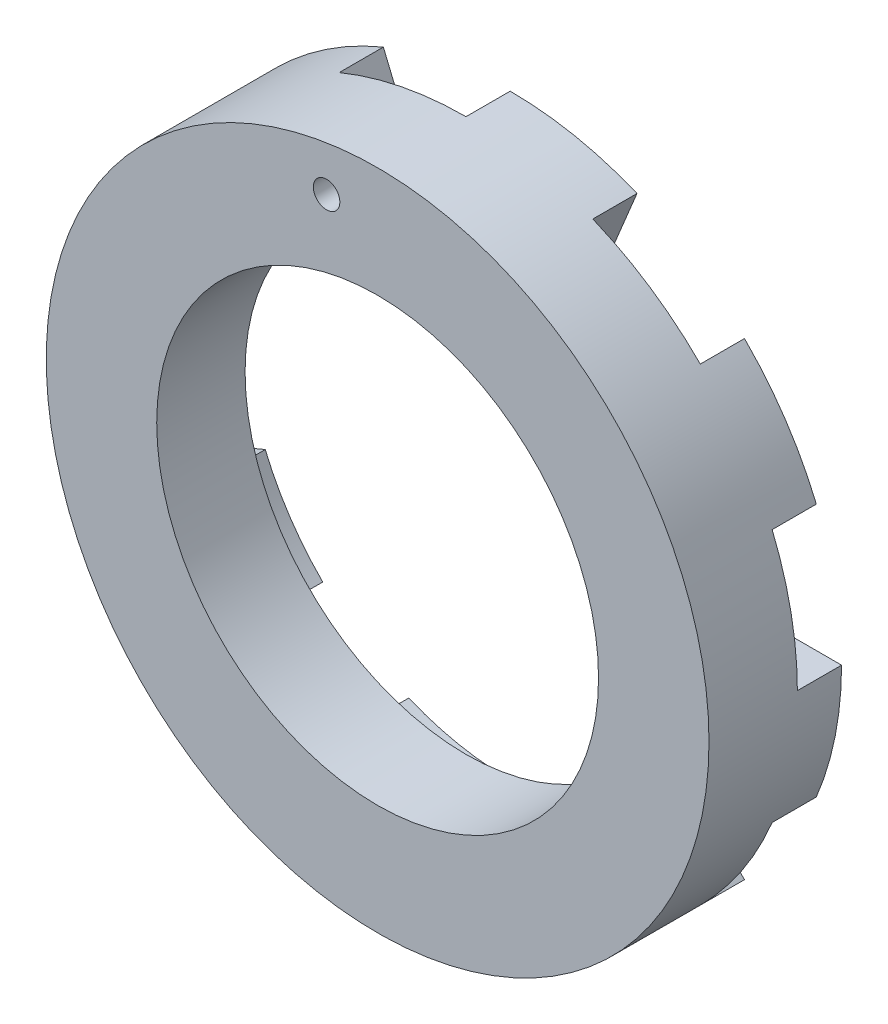
from build123d import *

# Parameters (mm, degrees)
SKETCH1_R           = 37.5
SKETCH1_R_2         = 25
BOSS_EXTRUDE1_DEPTH = 15
SKETCH2_R           = 30
CUT_EXTRUDE1_DEPTH  = 5
CUT_EXTRUDE2_DEPTH  = 5
SKETCH4_R           = 1.5
CUT_EXTRUDE3_DEPTH  = 10


with BuildPart() as part:
    # Sketch1 → Boss-Extrude1 (new body)
    with BuildSketch(Plane.XY):
        Circle(SKETCH1_R)
        Circle(SKETCH1_R_2, mode=Mode.SUBTRACT)
    extrude(amount=BOSS_EXTRUDE1_DEPTH)

    # Sketch2 → Cut-Extrude1 (cut)
    with BuildSketch(Plane(origin=(0, 0, 0), x_dir=(-1, 0, 0), z_dir=(0, 0, -1))):
        Circle(SKETCH2_R)
    extrude(amount=-CUT_EXTRUDE1_DEPTH, mode=Mode.SUBTRACT)

    # Sketch3 → Cut-Extrude2 (cut)
    with BuildSketch(Plane(origin=(0, 0, 0), x_dir=(-1, 0, 0), z_dir=(0, 0, -1))):
        with BuildLine():
            Line((0, 30), (0, 37.5))
            ThreePointArc((0, 37.5), (7.315887076, 36.779448015), (14.350628714, 34.645482469))
            Line((14.350628714, 34.645482469), (11.480502971, 27.716385975))
            ThreePointArc((11.480502971, 27.716385975), (5.85270966, 29.423558412), (0, 30))
        make_face()
        with BuildLine():
            Line((21.213203436, 21.213203436), (26.516504294, 26.516504294))
            ThreePointArc((26.516504294, 26.516504294), (31.180110461, 20.833883738), (34.645482469, 14.350628714))
            Line((34.645482469, 14.350628714), (27.716385975, 11.480502971))
            ThreePointArc((27.716385975, 11.480502971), (24.944088369, 16.667106991), (21.213203436, 21.213203436))
        make_face()
        with BuildLine():
            Line((30, 0), (37.5, 0))
            ThreePointArc((37.5, 0), (36.779448015, -7.315887076), (34.645482469, -14.350628714))
            Line((34.645482469, -14.350628714), (27.716385975, -11.480502971))
            ThreePointArc((27.716385975, -11.480502971), (29.423558412, -5.85270966), (30, 0))
        make_face()
        with BuildLine():
            Line((21.213203436, -21.213203436), (26.516504294, -26.516504294))
            ThreePointArc((26.516504294, -26.516504294), (20.833883738, -31.180110461), (14.350628714, -34.645482469))
            Line((14.350628714, -34.645482469), (11.480502971, -27.716385975))
            ThreePointArc((11.480502971, -27.716385975), (16.667106991, -24.944088369), (21.213203436, -21.213203436))
        make_face()
        with BuildLine():
            Line((0, -30), (0, -37.5))
            ThreePointArc((0, -37.5), (-7.315887076, -36.779448015), (-14.350628714, -34.645482469))
            Line((-14.350628714, -34.645482469), (-11.480502971, -27.716385975))
            ThreePointArc((-11.480502971, -27.716385975), (-5.85270966, -29.423558412), (0, -30))
        make_face()
        with BuildLine():
            Line((-21.213203436, -21.213203436), (-26.516504294, -26.516504294))
            ThreePointArc((-26.516504294, -26.516504294), (-31.180110461, -20.833883738), (-34.645482469, -14.350628714))
            Line((-34.645482469, -14.350628714), (-27.716385975, -11.480502971))
            ThreePointArc((-27.716385975, -11.480502971), (-24.944088369, -16.667106991), (-21.213203436, -21.213203436))
        make_face()
        with BuildLine():
            Line((-30, 0), (-37.5, 0))
            ThreePointArc((-37.5, 0), (-36.779448015, 7.315887076), (-34.645482469, 14.350628714))
            Line((-34.645482469, 14.350628714), (-27.716385975, 11.480502971))
            ThreePointArc((-27.716385975, 11.480502971), (-29.423558412, 5.85270966), (-30, 0))
        make_face()
        with BuildLine():
            Line((-21.213203436, 21.213203436), (-26.516504294, 26.516504294))
            ThreePointArc((-26.516504294, 26.516504294), (-20.833883738, 31.180110461), (-14.350628714, 34.645482469))
            Line((-14.350628714, 34.645482469), (-11.480502971, 27.716385975))
            ThreePointArc((-11.480502971, 27.716385975), (-16.667106991, 24.944088369), (-21.213203436, 21.213203436))
        make_face()
    extrude(amount=-CUT_EXTRUDE2_DEPTH, mode=Mode.SUBTRACT)

    # Sketch4 → Cut-Extrude3 (cut)
    with BuildSketch(Plane(origin=(0, 0, 5), x_dir=(-1, 0, 0), z_dir=(0, 0, -1))):
        with Locations((5.775719967, 31.982668101)):
            Circle(SKETCH4_R)
    extrude(amount=-CUT_EXTRUDE3_DEPTH, mode=Mode.SUBTRACT)


solid = part.part
